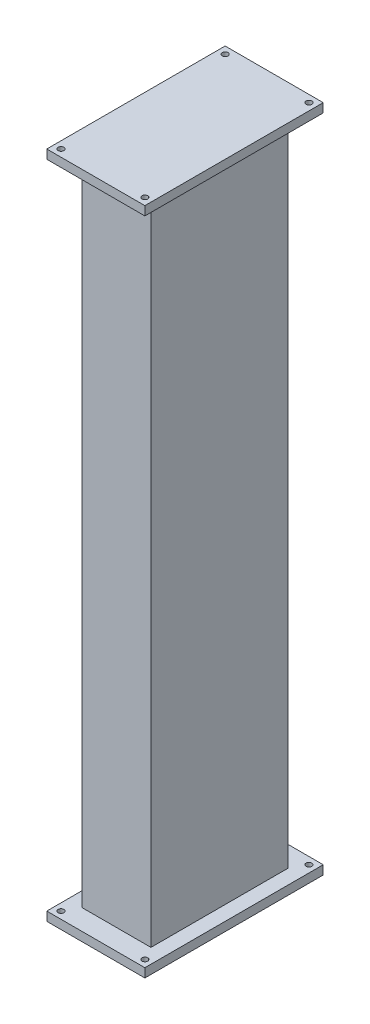
SolidWorks part; units mm, degrees
ref_plane "Front Plane" through (0, 0, 0) normal (0, 0, 1) x (1, 0, 0)
ref_plane "Top Plane" through (0, 0, 0) normal (0, 1, 0) x (1, 0, 0)
ref_plane "Right Plane" through (0, 0, 0) normal (1, 0, 0) x (0, 0, -1)
sketch "Sketch1" plane through (0, 0, 0) normal (0, 1, 0) x (1, 0, 0)
  line L1 (-55, -100) -> (55, -100)
  line L2 (-55, -100) -> (-55, 100)
  line L3 (-55, 100) -> (55, 100)
  line L4 (55, -100) -> (55, 100)
  line L5 (-55, -100) -> (55, 100) construction
  line L6 (-55, 100) -> (55, -100) construction
  line L7 (-47, -92) -> (47, -92) construction
  line L8 (-47, -92) -> (-47, 92) construction
  line L9 (-47, 92) -> (47, 92) construction
  line L10 (47, -92) -> (47, 92) construction
  line L11 (-47, -92) -> (47, 92) construction
  line L12 (-47, 92) -> (47, -92) construction
  circle A0 centre (-47, 92) radius 3.25
  circle A1 centre (47, 92) radius 3.25
  circle A2 centre (47, -92) radius 3.25
  circle A3 centre (-47, -92) radius 3.25
  point P0 (0, 0)
  point P6 (0, 0)
  dimension "D5" = 6.5
  dimension "D6" = 6.5
  dimension "D7" = 6.5
  dimension "D8" = 6.5
  dimension "D1" = 110
  dimension "D2" = 200
  dimension "D3" = 94
  dimension "D4" = 184
extrude "Boss-Extrude1" add sketch "Sketch1" along normal blind 10
sketch "Sketch2" plane through (0, 10, 0) normal (0, 1, 0) x (1, 0, 0)
  line L1 (-38.6724, -76.8778) -> (38.6724, -76.8778)
  line L2 (-38.6724, -76.8778) -> (-38.6724, 76.8778)
  line L3 (-38.6724, 76.8778) -> (38.6724, 76.8778)
  line L4 (38.6724, -76.8778) -> (38.6724, 76.8778)
  line L5 (-38.6724, -76.8778) -> (38.6724, 76.8778) construction
  line L6 (-38.6724, 76.8778) -> (38.6724, -76.8778) construction
  point P0 (0, 0)
extrude "Boss-Extrude2" add sketch "Sketch2" along normal blind 730
sketch "Sketch4" plane through (0, 740, 0) normal (0, 1, 0) x (1, 0, 0)
  line L0 (-55, -100) -> (55, -100)
  line L1 (-55, -100) -> (-55, 100)
  line L2 (-55, 100) -> (55, 100)
  line L3 (55, -100) -> (55, 100)
  line L4 (-55, -100) -> (55, 100) construction
  line L5 (-55, 100) -> (55, -100) construction
  line L6 (-47, -92) -> (47, -92) construction
  line L7 (-47, -92) -> (-47, 92) construction
  line L8 (-47, 92) -> (47, 92) construction
  line L9 (47, -92) -> (47, 92) construction
  line L10 (-47, -92) -> (47, 92) construction
  line L11 (-47, 92) -> (47, -92) construction
  circle A0 centre (-47, 92) radius 3.25
  circle A1 centre (47, 92) radius 3.25
  circle A2 centre (47, -92) radius 3.25
  circle A3 centre (-47, -92) radius 3.25
  point P0 (0, 0)
  point P5 (0, 0)
  dimension "D4" = 6.5
  dimension "D5" = 6.5
  dimension "D6" = 6.5
  dimension "D7" = 6.5
  dimension "D1" = 110
  dimension "D2" = 200
  dimension "D3" = 94
extrude "Boss-Extrude4" add sketch "Sketch4" along normal blind 10
